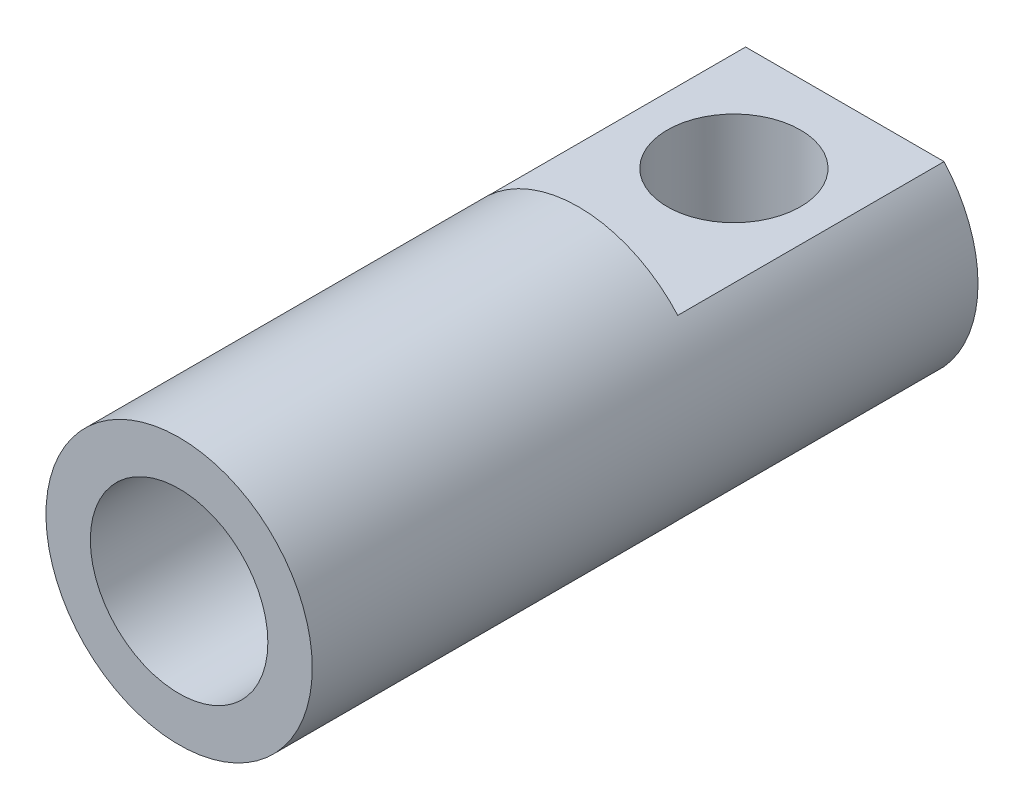
SolidWorks part; units mm, degrees
ref_plane "Front Plane" through (0, 0, 0) normal (0, 0, 1) x (1, 0, 0)
ref_plane "Top Plane" through (0, 0, 0) normal (0, 1, 0) x (1, 0, 0)
ref_plane "Right Plane" through (0, 0, 0) normal (1, 0, 0) x (0, 0, -1)
sketch "Sketch1" plane through (0, 0, 0) normal (0, 0, 1) x (1, 0, 0)
  circle A0 centre (0, 0) radius 6
  dimension "D1" = 12
extrude "Boss-Extrude1" add sketch "Sketch1" along normal blind 30
sketch "Sketch2" plane through (0, 0, 0) normal (0, 1, 0) x (1, 0, 0)
  line L0 (6, 0) -> (-6, 0) construction
  line L1 (-10.8799, 3.3091) -> (11.5832, 3.3091)
  line L2 (-10.8799, 3.3091) -> (-10.8799, -12)
  line L3 (-10.8799, -12) -> (11.5832, -12)
  line L4 (11.5832, 3.3091) -> (11.5832, -12)
  dimension "D1" = 12
extrude "Cut-Extrude1" cut sketch "Sketch2" against normal blind 10 from offset 4 offset against normal yes
mirror "Mirror1" about plane through (0, 0, 0) normal (0, 1, 0) of "Cut-Extrude1"
sketch "Sketch3" plane through (0, -4, 0) normal (0, -1, 0) x (1, 0, 0)
  line L0 (4.4721, 0) -> (-4.4721, 0) construction
  circle A0 centre (0, 5) radius 3
  dimension "D1" = 6
  dimension "D2" = 5
extrude "Cut-Extrude2" cut sketch "Sketch3" against normal through all both and the other way through all
sketch "Sketch4" plane through (0, 0, 30) normal (0, 0, 1) x (1, 0, 0)
  circle A0 centre (0, 0) radius 4
  dimension "D1" = 8
extrude "Cut-Extrude3" cut sketch "Sketch4" against normal blind 10
